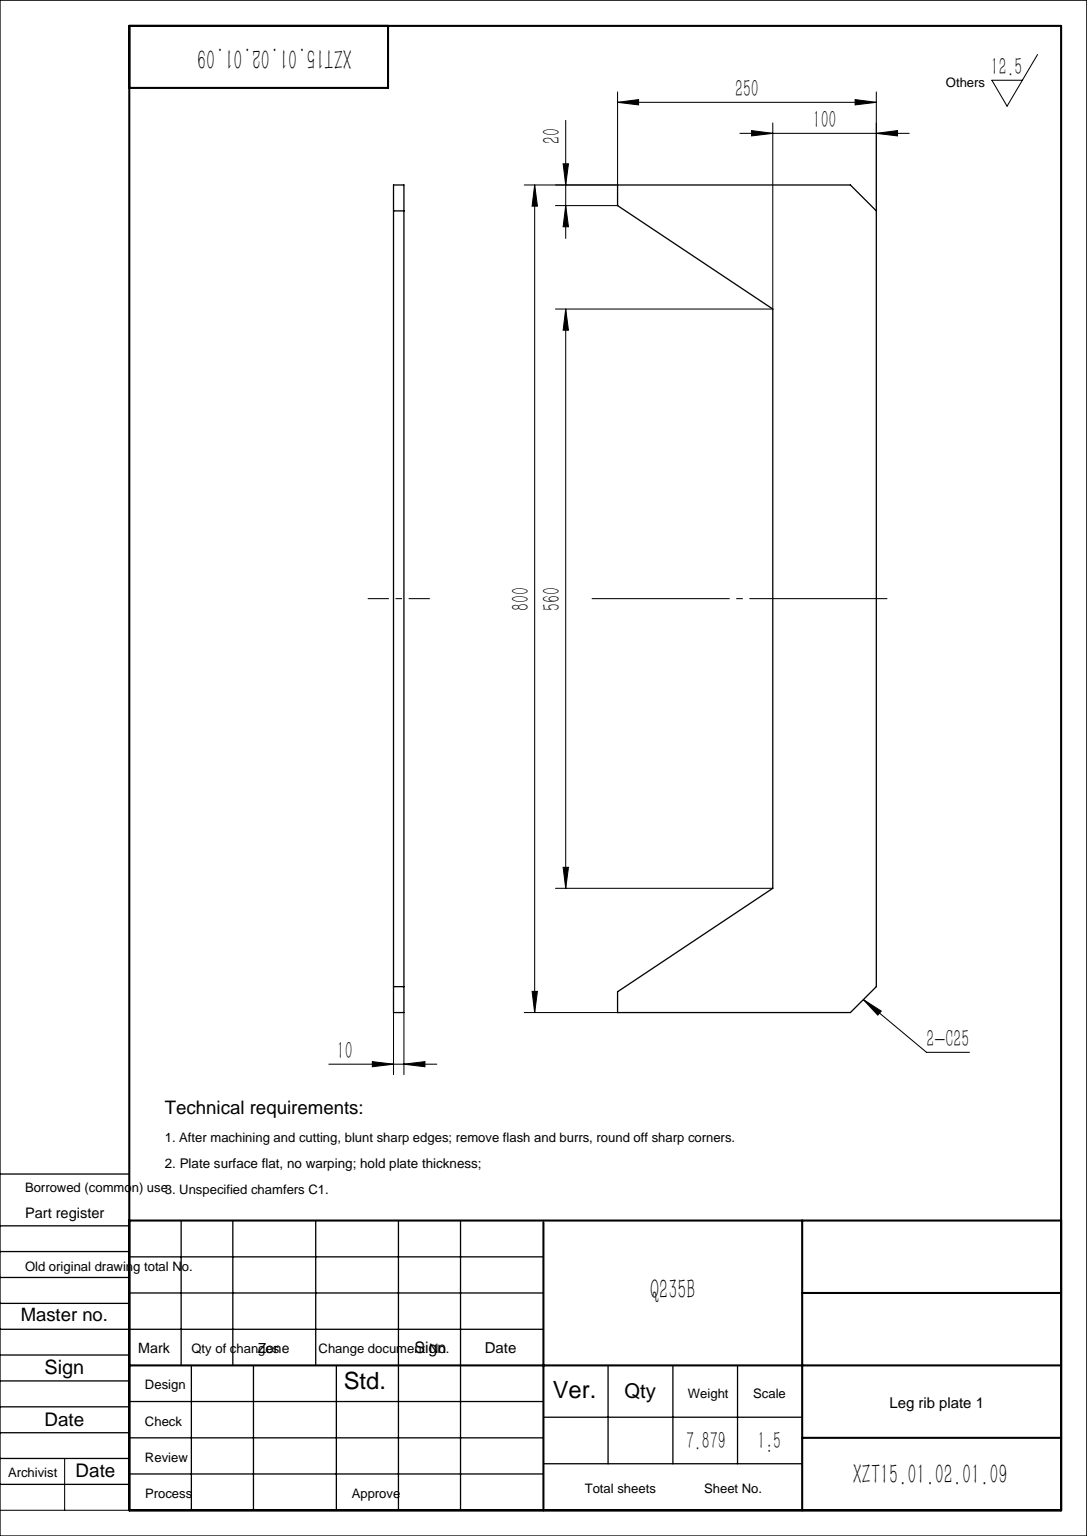
SolidWorks part; units mm, degrees
material "Q235B"
ref_plane "Front Plane" through (0, 0, 0) normal (0, 0, 1) x (1, 0, 0)
ref_plane "Top Plane" through (0, 0, 0) normal (0, 1, 0) x (1, 0, 0)
ref_plane "Right Plane" through (0, 0, 0) normal (1, 0, 0) x (0, 0, -1)
sketch "Sketch1" plane through (0, 0, 0) normal (0, 0, 1) x (1, 0, 0)
  line L0 (0, -280) -> (0, 280)
  line L1 (0, 280) -> (-150, 380)
  line L2 (-150, 380) -> (-150, 400)
  line L3 (-150, 400) -> (100, 400)
  line L4 (100, 400) -> (100, -400)
  line L5 (100, 0) -> (-0.2875, 0) construction
  line L6 (-150, -400) -> (100, -400)
  line L7 (-150, -380) -> (-150, -400)
  line L8 (0, -280) -> (-150, -380)
  point P12 (0, 0)
  dimension "D1" = 800
  dimension "D2" = 560
  dimension "D3" = 20
  dimension "D4" = 250
  dimension "D5" = 100
extrude "Boss-Extrude1" add sketch "Sketch1" along normal mid plane 10
chamfer "Chamfer1" distance 25 angle 45 2 edges at (100, -400, 0) (100, 400, 0)
